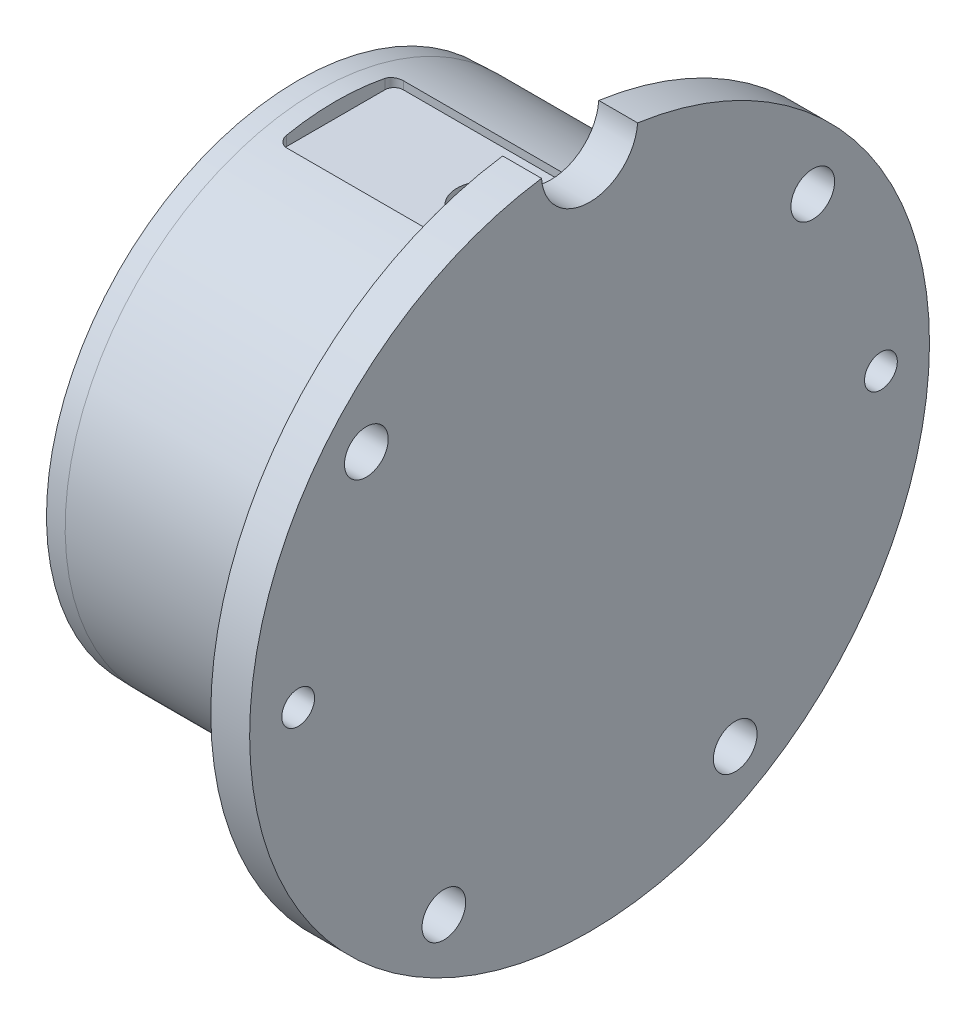
SolidWorks part; units mm, degrees
material "灰铸铁"
ref_plane "Front Plane" through (0, 0, 0) normal (0, 0, 1) x (1, 0, 0)
ref_plane "Top Plane" through (0, 0, 0) normal (0, 1, 0) x (1, 0, 0)
ref_plane "Right Plane" through (0, 0, 0) normal (1, 0, 0) x (0, 0, -1)
sketch "Sketch1" plane through (0, 0, 0) normal (0, 0, 1) x (1, 0, 0)
  line L0 (0, 0) -> (-95.25, 0) construction
  line L1 (-95.25, 70.62) -> (-95.25, 82.2956)
  line L2 (-88.9, 82.5373) -> (-12.7, 82.5373)
  line L3 (-12.7, 82.5373) -> (-12.7, 111.125)
  line L4 (-12.7, 111.125) -> (0, 111.125)
  line L5 (0, 111.125) -> (0, 0)
  line L6 (0, 0) -> (-24.2804, 0)
  line L7 (-24.2804, 0) -> (-24.2804, 65.913)
  line L8 (-24.2804, 65.913) -> (-40.0304, 65.913)
  line L9 (-40.0304, 65.913) -> (-40.0304, 70.0075)
  line L10 (-40.0304, 70.0075) -> (-88.4682, 70.0075)
  line L11 (-40.0304, -70.0075) -> (-68.9301, -70.0075) construction
  line L12 (-40.0304, -65.913) -> (-40.0304, -70.0075) construction
  line L13 (-24.2804, -65.913) -> (-40.0304, -65.913) construction
  line L14 (-12.7, -111.125) -> (0, -111.125) construction
  line L15 (-12.7, -82.5373) -> (-12.7, -111.125) construction
  line L16 (-68.9301, -82.5373) -> (-12.7, -82.5373) construction
  line L17 (-68.9301, -70.0075) -> (-68.9301, -82.5373) construction
  line L18 (-91.5162, 70.0075) -> (-91.5162, 73.279)
  line L19 (-91.5162, 73.279) -> (-88.4682, 73.279)
  line L20 (-88.4682, 73.279) -> (-88.4682, 70.0075)
  line L21 (-91.5162, 70.0075) -> (-92.964, 70.0075)
  line L22 (-92.964, 70.0075) -> (-95.25, 70.62)
  line L23 (-91.5162, -73.279) -> (-88.4682, -73.279) construction
  line L24 (-92.964, -70.0075) -> (-95.25, -70.62) construction
  line L25 (-95.25, 82.2956) -> (-88.9, 82.5373)
  line L26 (-95.25, -82.2956) -> (-88.9, -82.5373) construction
  dimension "D1" = 165.0746
  dimension "D2" = 140.015
  dimension "D3" = 15
  dimension "D4" = 146.558
  dimension "D5" = 131.826
  dimension "D6" = 222.25
  dimension "D7" = 6.35
  dimension "D8" = 164.5912
  dimension "D9" = 12.7
  dimension "D10" = 82.55
  dimension "D11" = 27.3304
  dimension "D12" = 15.75
  dimension "D13" = 3.048
  dimension "D14" = 51.4858
  dimension "D15" = 2.286
revolve "Revolve1" add sketch "Sketch1" angle 360 about L0
hole_wizard "9/16 (0.5625) Diameter Hole1" positions "Sketch4" profile "Sketch3" hole size "9/16" standard "Ansi Inch" end condition up to next
sketch "Sketch4" plane through (0, 0, 0) normal (1, 0, 0) x (0, 0, -1)
  line L0 (0, 0) -> (0, 106.2938) construction
  line L2 (0, 0) -> (74.1658, 0) construction
  point P0 (-72.9742, 61.2154)
  point P2 (72.9742, 61.2154)
  point P4 (-47.625, -82.4992)
  point P6 (47.625, -82.4992)
  dimension "D1" = 72.9742
  dimension "D2" = 61.2154
  dimension "D3" = 82.4992
  dimension "D4" = 47.625
sketch "Sketch3" plane through (0, 61.2154, 72.9742) normal (0, 1, 0) x (0, 0, -1)
  line L0 (0, 0) -> (0, 12.7)
  line L1 (0, 12.7) -> (7.1437, 12.7)
  line L2 (7.1437, 12.7) -> (7.1437, 0)
  line L5 (7.1437, 0) -> (0, 0)
  line L11 (0, -6.35) -> (0, 107.95) construction
  dimension "通孔孔直径" = 14.2875
  dimension "通孔孔深度" = 12.7
hole_wizard "1/2-13 Tapped Hole1" positions "Sketch6" profile "Sketch7" tap size "1/2-13" standard "Ansi Inch" end condition up to next
sketch "Sketch6" plane through (0, 0, 0) normal (1, 0, 0) x (0, 0, -1)
  line L0 (0, 0) -> (-95.25, 0) construction
  line L1 (0, 0) -> (0, 36.1076) construction
  point P2 (-95.25, 0)
  point P8 (95.25, 0)
  dimension "D1" = 95.25
sketch "Sketch7" plane through (0, 0, 95.25) normal (0, 1, 0) x (0, 0, -1)
  line L0 (0, 0) -> (0, 12.7)
  line L1 (0, 12.7) -> (5.3581, 12.7)
  line L2 (5.3581, 12.7) -> (5.3581, 0)
  line L5 (5.3581, 0) -> (0, 0)
  line L11 (0, -6.35) -> (0, 107.95) construction
  dimension "螺纹线主直径" = 10.7163
  dimension "通孔螺纹孔钻头深度" = 12.7
sketch "Sketch8" plane through (0, 0, 0) normal (0, 1, 0) x (1, 0, 0)
  line L0 (-24.2804, 19.05) -> (-82.9544, 19.05)
  line L2 (-82.9544, 19.05) -> (-82.9544, -19.05)
  line L3 (-82.9544, -19.05) -> (-24.2804, -19.05)
  line L4 (-24.2804, 19.05) -> (-24.2804, -19.05)
  line L5 (0, 0) -> (-82.9544, 0) construction
  line L6 (-24.2804, 65.913) -> (-24.2804, -65.913) construction
  dimension "D1" = 58.674
  dimension "D2" = 38.1
extrude "Extrude1" cut sketch "Sketch8" against normal offset from surface (22.276 mm away) 77.724 from offset 100
sketch "Sketch9" plane through (0, 77.724, 0) normal (0, 1, 0) x (1, 0, 0)
  line L2 (0, 0) -> (-33.8054, 0) construction
  line L9 (-24.2804, 19.05) -> (-24.2804, -19.05) construction
  circle A0 centre (-33.8054, 0) radius 9.525
  dimension "D1" = 19.05
extrude "Extrude2" cut sketch "Sketch9" against normal up to surface (12.5029 mm away)
fillet "Fillet1" radius 3 2 edges at (-82.9544, 79.0164, 19.05) (-82.9544, 79.0164, -19.05)
sketch "Sketch10" plane through (0, 0, 0) normal (1, 0, 0) x (0, 0, -1)
  line L0 (0, 0) -> (0, 111.125) construction
  circle A0 centre (0, 0) radius 111.125 construction
  arc A1 (-15.7084, 110.0091) -> (15.7084, 110.0091) centre (0, 111.125) ccw
  arc A2 (15.7084, 110.0091) -> (-15.7084, 110.0091) centre (0, 0) ccw
  dimension "D1" = 15.748
extrude "Extrude3" cut sketch "Sketch10" against normal up to next
